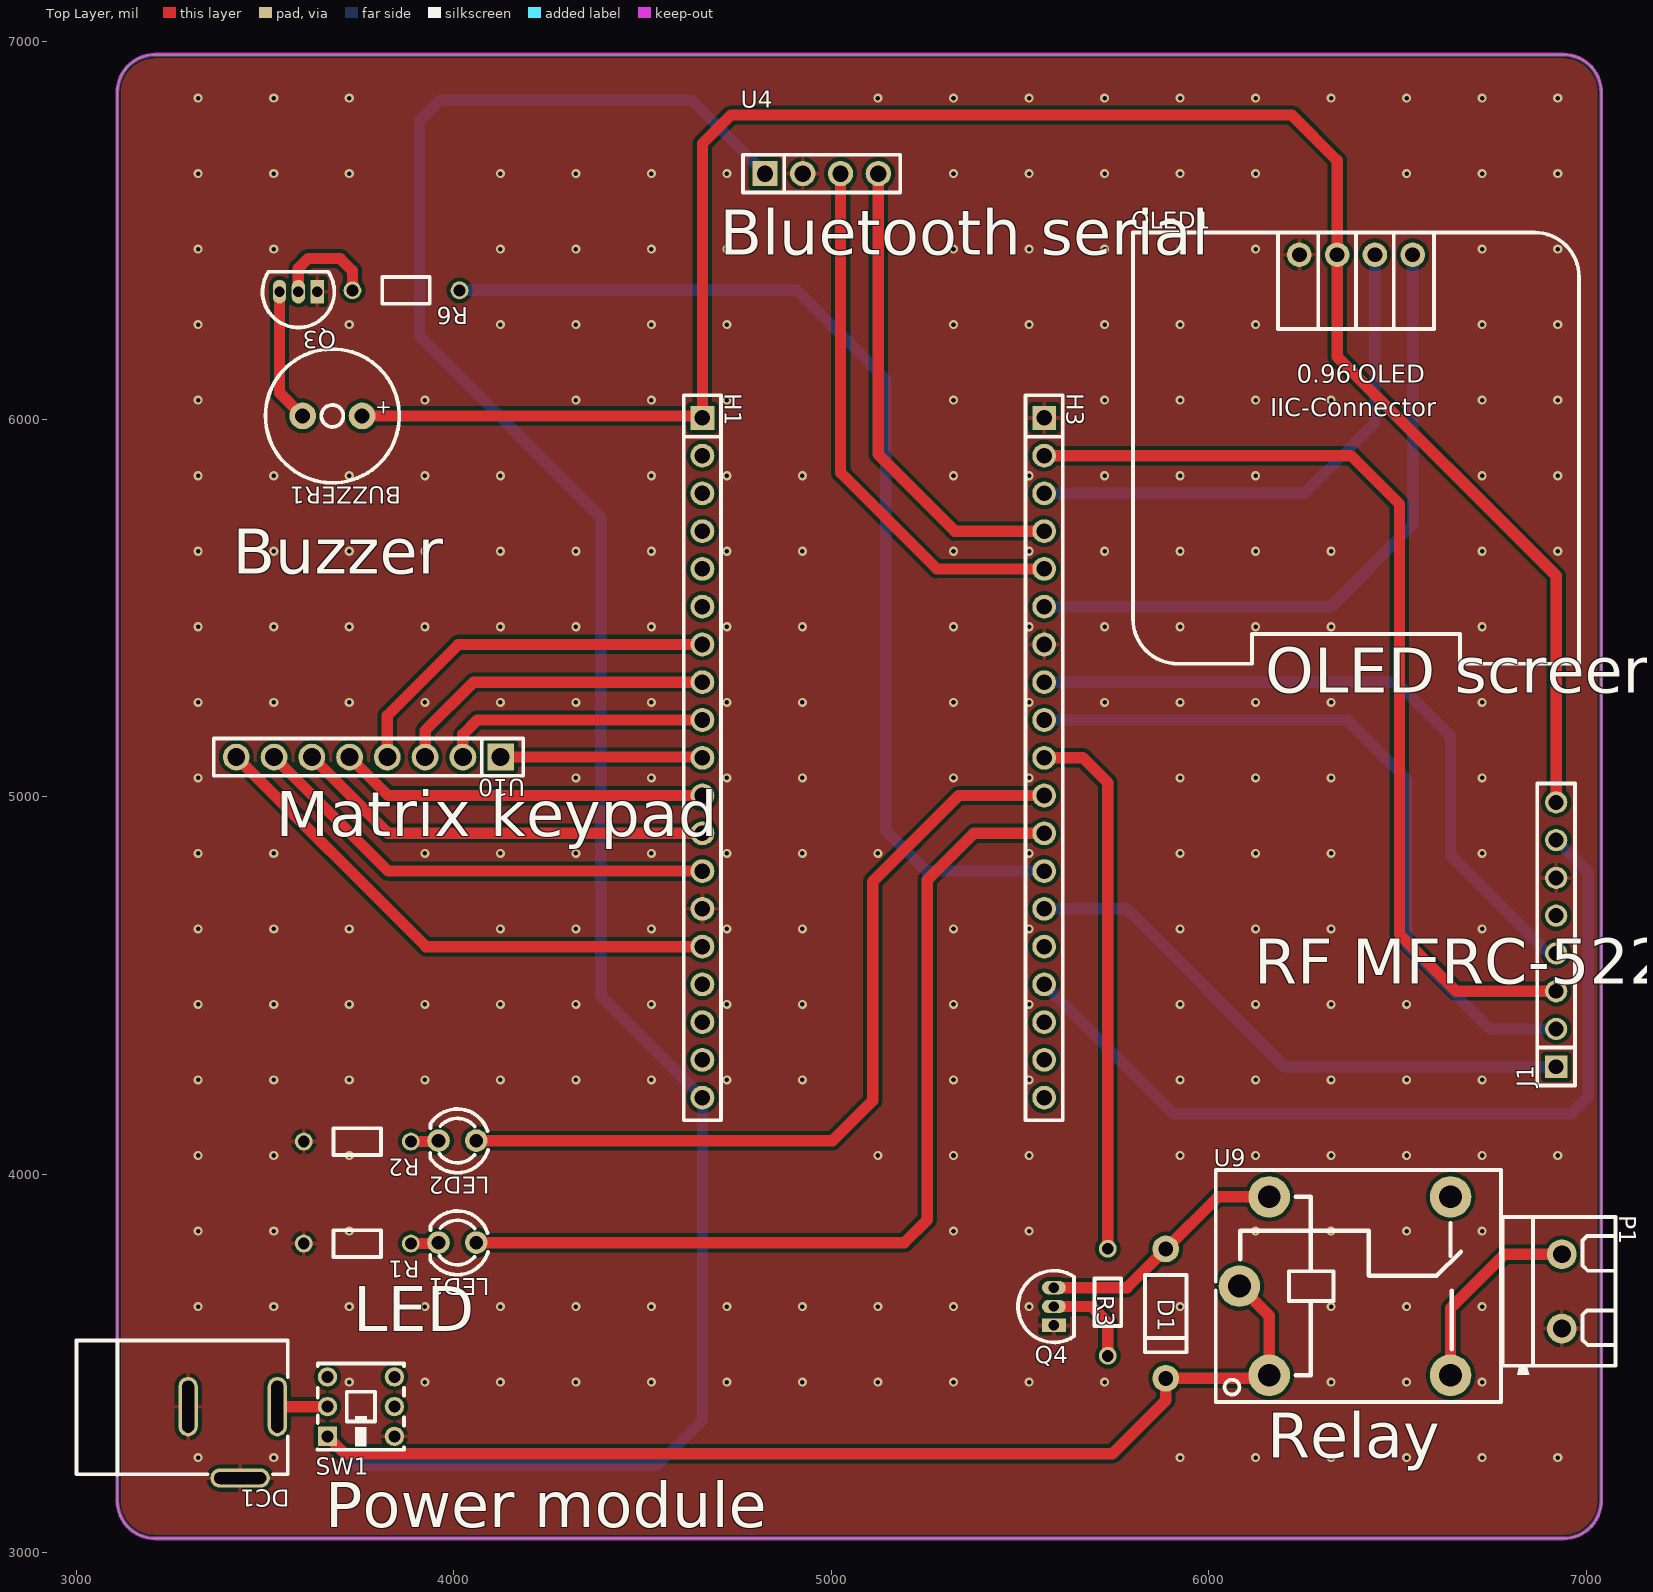
[diagram p0: Top Layer view]
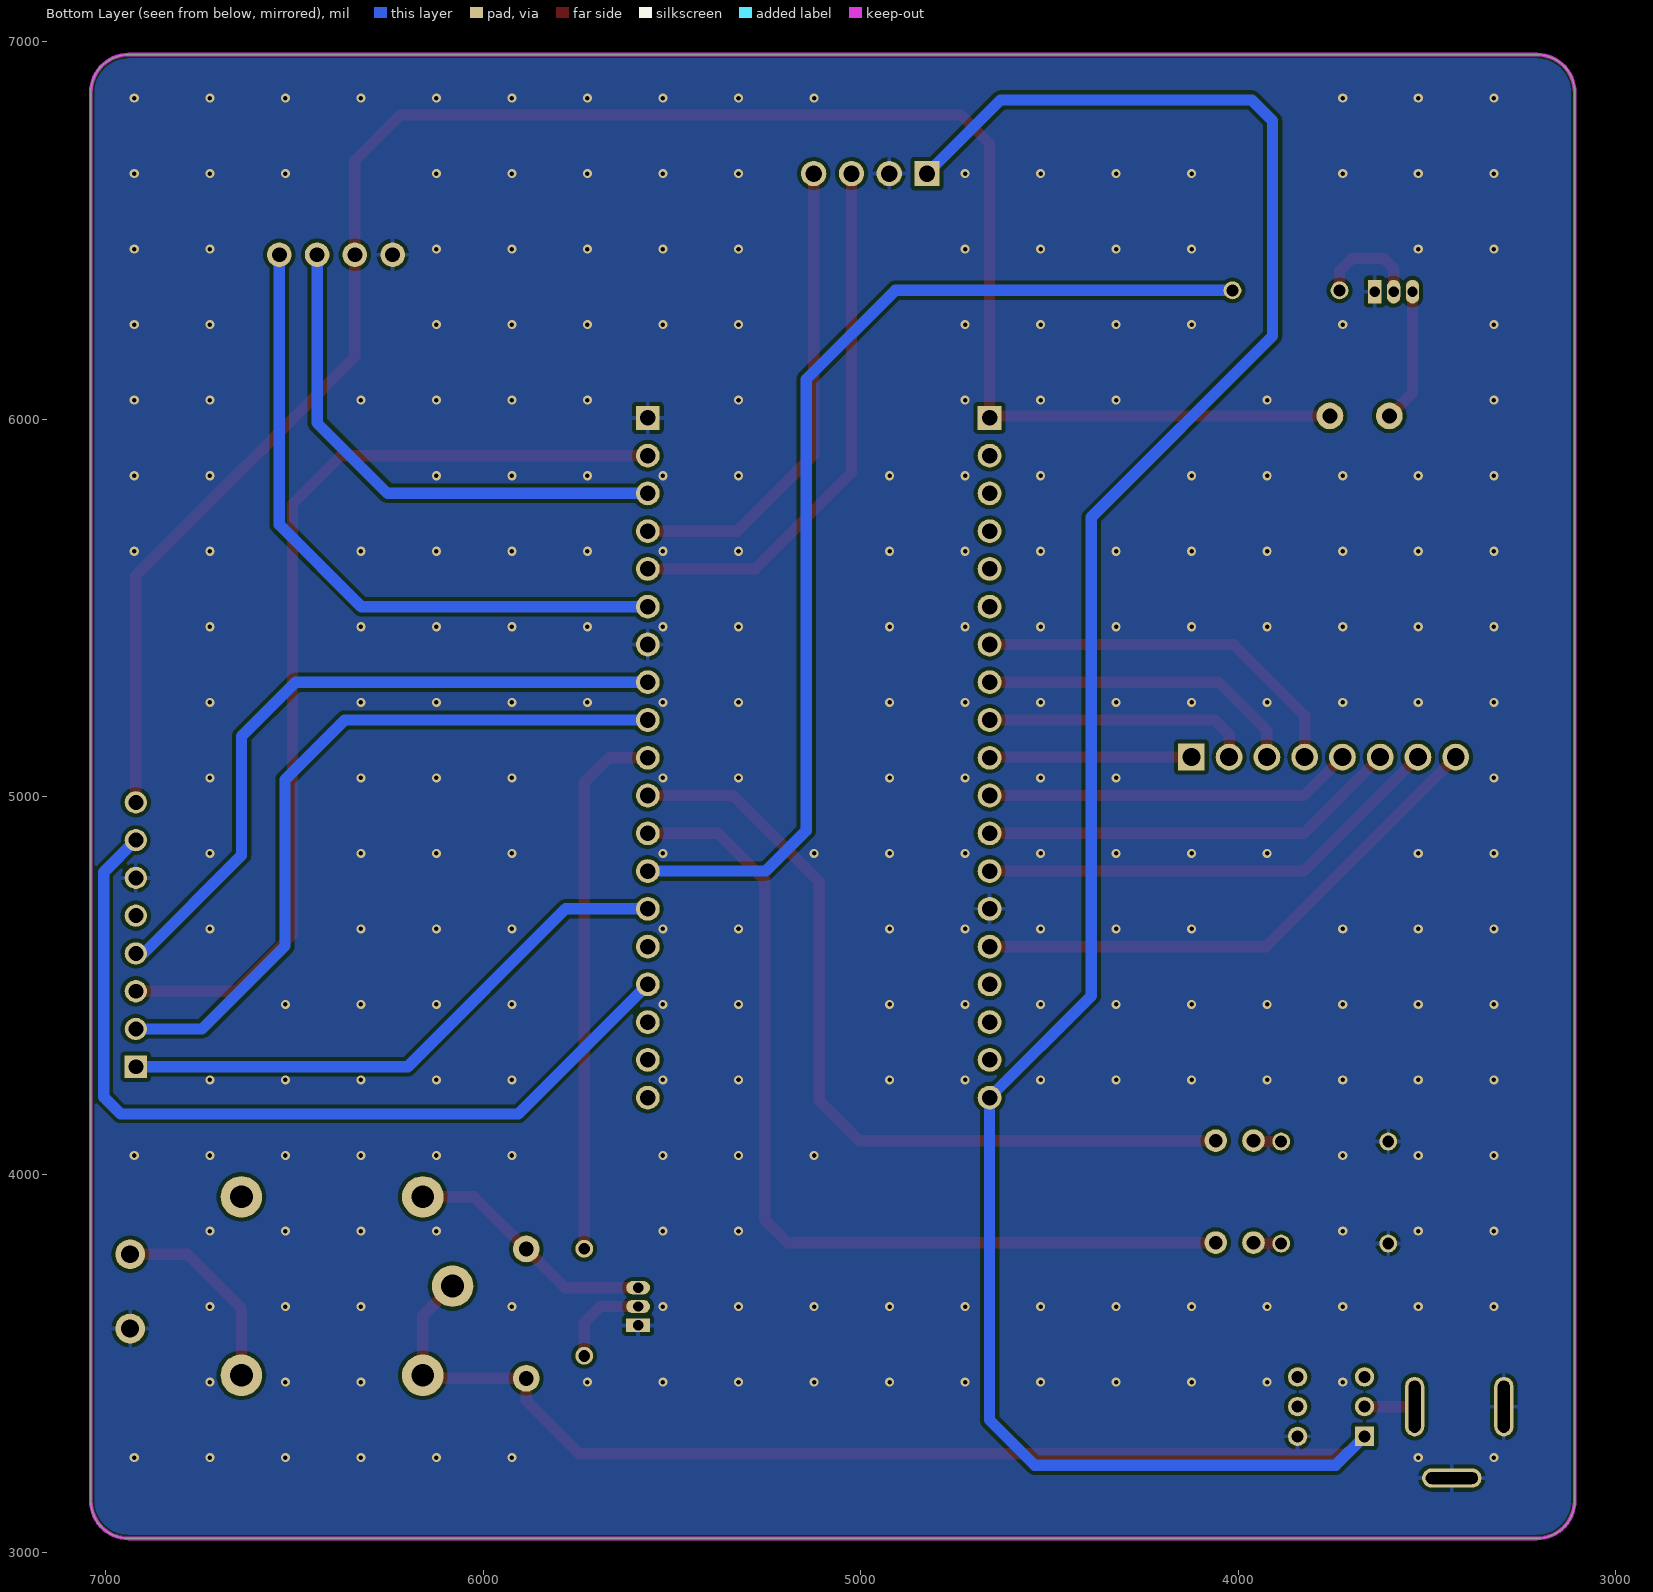
[diagram p1: Bottom Layer view, seen from below]
# Altium PCB MISC89084.pcbdoc
Units mil, origin at the board's own origin, x right, y up, seen from the top; angles counter-clockwise.
Board outline 3929.13 x 3929.13 mil, 2 copper layers (Top Layer, Bottom Layer), stack 62.206 mil thick; 20 components, 44 nets, 100 pads, 259 vias.

## Layer stack, top to bottom
Top Solder Mask Layer: solder mask 0.394, Dk 3.3
Top Layer: signal copper 1.379
Dielectric1: surface 59.449, FR4, Dk 4.5
Bottom Layer: signal copper 1.378
Bottom Solder Mask Layer: solder mask 0.394, Dk 3.3

## Board outline
3209.4,6965 ccw(c3209.4,6865) 3109.4,6865 3109.4,3135.87 ccw(c3209.4,3135.87) 3209.4,3035.87 6938.53,3035.87 ccw(c6938.53,3135.87) 7038.53,3135.87 7038.53,6865 ccw(c6938.53,6865) 6938.53,6965

## Design rules (kind name [scope] priority, off if disabled: settings)
BoardOutlineClearance copperThickness2oz_1 [All] p2 off: genericclearance=7.99 ignorepadtopadclearanceinfootprint=FALSE except(0: Arc-SplitContinuation Track-SplitContinuation SMDPad-SplitContinuation THPad-SplitContinuation Via-SplitContinuation Fill-SplitContinuation Region-SplitContinuation Poly-SplitContinuation Text-SplitContinuation Hole-SplitContinuation; 5.98: Arc-CutoutEdge Track-CutoutEdge SMDPad-CutoutEdge THPad-CutoutEdge Via-CutoutEdge Text-CutoutEdge; 6.9: Hole-OutlineEdge Hole-CutoutEdge; 10: Poly-OutlineEdge Poly-CutoutEdge; 11.81: Arc-OutlineEdge Track-OutlineEdge SMDPad-OutlineEdge THPad-OutlineEdge Via-OutlineEdge Fill-OutlineEdge Region-OutlineEdge Text-OutlineEdge Fill-CutoutEdge Region-CutoutEdge)
BoardOutlineClearance Plane_innerPlane_1 [All] p4 off: genericclearance=4.02 ignorepadtopadclearanceinfootprint=FALSE except(0: Arc-SplitContinuation Track-SplitContinuation SMDPad-SplitContinuation THPad-SplitContinuation Via-SplitContinuation Fill-SplitContinuation Region-SplitContinuation Poly-SplitContinuation Text-SplitContinuation Hole-SplitContinuation; 5.98: Arc-CutoutEdge Track-CutoutEdge SMDPad-CutoutEdge THPad-CutoutEdge Via-CutoutEdge Text-CutoutEdge; 6.9: Hole-OutlineEdge Hole-CutoutEdge; 10: Poly-OutlineEdge Poly-CutoutEdge; 11.81: Arc-OutlineEdge Track-OutlineEdge SMDPad-OutlineEdge THPad-OutlineEdge Via-OutlineEdge Fill-OutlineEdge Region-OutlineEdge Text-OutlineEdge Fill-CutoutEdge Region-CutoutEdge)
BoardOutlineClearance Copper_copperRegion_1 [All] p6 off: genericclearance=4.02 ignorepadtopadclearanceinfootprint=FALSE except(0: Arc-SplitContinuation Track-SplitContinuation SMDPad-SplitContinuation THPad-SplitContinuation Via-SplitContinuation Fill-SplitContinuation Region-SplitContinuation Poly-SplitContinuation Text-SplitContinuation Hole-SplitContinuation; 5.98: Arc-CutoutEdge Track-CutoutEdge SMDPad-CutoutEdge THPad-CutoutEdge Via-CutoutEdge Text-CutoutEdge; 6.9: Hole-OutlineEdge Hole-CutoutEdge; 10: Poly-OutlineEdge Poly-CutoutEdge; 11.81: Arc-OutlineEdge Track-OutlineEdge SMDPad-OutlineEdge THPad-OutlineEdge Via-OutlineEdge Fill-OutlineEdge Region-OutlineEdge Text-OutlineEdge Fill-CutoutEdge Region-CutoutEdge)
BoardOutlineClearance copperThickness1oz_1 [All] p8: genericclearance=4.02 ignorepadtopadclearanceinfootprint=FALSE except(0: Arc-SplitContinuation Track-SplitContinuation SMDPad-SplitContinuation THPad-SplitContinuation Via-SplitContinuation Fill-SplitContinuation Region-SplitContinuation Poly-SplitContinuation Text-SplitContinuation Hole-SplitContinuation; 5.98: Arc-CutoutEdge Track-CutoutEdge SMDPad-CutoutEdge THPad-CutoutEdge Via-CutoutEdge Text-CutoutEdge; 6.9: Hole-OutlineEdge Hole-CutoutEdge; 10: Poly-OutlineEdge Poly-CutoutEdge; 11.81: Arc-OutlineEdge Track-OutlineEdge SMDPad-OutlineEdge THPad-OutlineEdge Via-OutlineEdge Fill-OutlineEdge Region-OutlineEdge Text-OutlineEdge Fill-CutoutEdge Region-CutoutEdge)
Clearance copperThickness2oz [All] p1 off: gap=7.99 ignorepadtopadclearanceinfootprint=FALSE except(5.98: SMDPad-Track SMDPad-SMDPad THPad-Track SMDPad-THPad THPad-THPad Track-Via SMDPad-Via THPad-Via Via-Via Fill-SMDPad Region-SMDPad Fill-THPad Region-THPad Fill-Via Region-Via Fill-Fill Fill-Region Region-Region Arc-Track Arc-SMDPad Arc-THPad Arc-Via Fill-Arc Region-Arc Arc-Arc Text-Track SMDPad-Text Text-THPad Text-Via Fill-Text Region-Text Arc-Text Text-Text; 6.9: Hole-Track Hole-SMDPad Hole-THPad Hole-Via Fill-Hole Region-Hole Hole-Arc Hole-Text; 10: Poly-Track Poly-SMDPad Poly-THPad Poly-Via Poly-Fill Poly-Region Poly-Poly Poly-Arc Poly-Text Poly-Hole; 11.81: Fill-Track Region-Track)
Clearance Plane_innerPlane [All] p3 off: gap=4.02 ignorepadtopadclearanceinfootprint=FALSE except(5.98: SMDPad-Track SMDPad-SMDPad THPad-Track SMDPad-THPad THPad-THPad Track-Via SMDPad-Via THPad-Via Via-Via Fill-SMDPad Region-SMDPad Fill-THPad Region-THPad Fill-Via Region-Via Fill-Fill Fill-Region Region-Region Arc-Track Arc-SMDPad Arc-THPad Arc-Via Fill-Arc Region-Arc Arc-Arc Text-Track SMDPad-Text Text-THPad Text-Via Fill-Text Region-Text Arc-Text Text-Text; 6.9: Hole-Track Hole-SMDPad Hole-THPad Hole-Via Fill-Hole Region-Hole Hole-Arc Hole-Text; 10: Poly-Track Poly-SMDPad Poly-THPad Poly-Via Poly-Fill Poly-Region Poly-Poly Poly-Arc Poly-Text Poly-Hole; 11.81: Fill-Track Region-Track)
Clearance Copper_copperRegion [All] p5 off: gap=4.02 ignorepadtopadclearanceinfootprint=FALSE except(5.98: SMDPad-Track SMDPad-SMDPad THPad-Track SMDPad-THPad THPad-THPad Track-Via SMDPad-Via THPad-Via Via-Via Fill-SMDPad Region-SMDPad Fill-THPad Region-THPad Fill-Via Region-Via Fill-Fill Fill-Region Region-Region Arc-Track Arc-SMDPad Arc-THPad Arc-Via Fill-Arc Region-Arc Arc-Arc Text-Track SMDPad-Text Text-THPad Text-Via Fill-Text Region-Text Arc-Text Text-Text; 6.9: Hole-Track Hole-SMDPad Hole-THPad Hole-Via Fill-Hole Region-Hole Hole-Arc Hole-Text; 10: Poly-Track Poly-SMDPad Poly-THPad Poly-Via Poly-Fill Poly-Region Poly-Poly Poly-Arc Poly-Text Poly-Hole; 11.81: Fill-Track Region-Track)
Clearance copperThickness1oz [All] p7: gap=4.02 ignorepadtopadclearanceinfootprint=FALSE except(5.98: SMDPad-Track SMDPad-SMDPad THPad-Track SMDPad-THPad THPad-THPad Track-Via SMDPad-Via THPad-Via Via-Via Fill-SMDPad Region-SMDPad Fill-THPad Region-THPad Fill-Via Region-Via Fill-Fill Fill-Region Region-Region Arc-Track Arc-SMDPad Arc-THPad Arc-Via Fill-Arc Region-Arc Arc-Arc Text-Track SMDPad-Text Text-THPad Text-Via Fill-Text Region-Text Arc-Text Text-Text; 6.9: Hole-Track Hole-SMDPad Hole-THPad Hole-Via Fill-Hole Region-Hole Hole-Arc Hole-Text; 10: Poly-Track Poly-SMDPad Poly-THPad Poly-Via Poly-Fill Poly-Region Poly-Poly Poly-Arc Poly-Text Poly-Hole; 11.81: Fill-Track Region-Track)
DiffPairsRouting differentialPair [All] p1: maxlimit=6 minlimit=6 mostfreqgap=6 toplayer_minwidth=5 toplayer_prefwidth=10 toplayer_maxwidth=100 toplayer_mingap=6 toplayer_prefgap=6 toplayer_maxgap=6 bottomlayer_minwidth=5 bottomlayer_prefwidth=10 bottomlayer_maxwidth=100 bottomlayer_mingap=6 bottomlayer_prefgap=6 bottomlayer_maxgap=6 maxuncoupledlength=10
HoleToHoleClearance otherClearance [All] p1: gap=11.81 allowstackedmicrovias=TRUE
Length netLength [All] p1: minlimit=0 maxlimit=0
PasteMaskExpansion pasteMaskExpansion [All] p1: expansion=0
PlaneConnect innerPlane [All] p1: planeconnectstyle=Relief reliefexpansion=20 reliefentries=4 reliefconductorwidth=10 reliefairgap=10
PolygonConnect copperRegion [All] p1: connectstyle=Relief reliefconductorwidth=10 reliefentries=4 polygonreliefangle="90 Angle" airgapwidth=10 via.connectstyle=Relief via.reliefconductorwidth=10 via.reliefentries=4 via.polygonreliefangle="90 Angle" via.airgapwidth=10
RoutingVias viaSize [All] p1: holewidth=12.01 width=24.02 viastyle="Through Hole" minholewidth=11.81 minwidth=19.68 maxholewidth=248.03 maxwidth=393.7
SolderMaskExpansion solderMaskExpansion [IsVia] p1: expansion=-1000 istentingtop=TRUE
SolderMaskExpansion solderMaskExpansion [All] p2: expansion=2 istentingtop=FALSE
Width copperThickness2oz_2 [All] p1 off: maxlimit=100 minlimit=8 preferedwidth=10
Width copperThickness1oz_2 [All] p2: maxlimit=100 minlimit=5 preferedwidth=10

## Components (designator, comment, footprint, x,y, rotation, side; value= is the part's Value field where it differs from the comment)
BUZZER1 "2.7kHz" BUZ-TH_BD9.0-P4.00-D0.6-FD 3678.79,6008.3 r180 top
D1 "" DO_1N4007 5885.61,3631.17 r90 top
DC1 "" DC-2.0 3410,3395.3 r180 top
H1 "C2897382" HDR-TH_19P-P2.54-V-F 4658.71,5103.13 r270 top
H3 "C2897382" HDR-TH_19P-P2.54-V-F 5563.71,5103.13 r270 top
J1 "" HDR-TH_8P-P2.54-V-M 6919.4,4635 r90 top
LED1 "" LED_TH-3mm 4009.8,3819.31 r180 top
LED2 "" LED_TH-3mm 4009.8,4089.31 r180 top
OLED1 "" 0.96OLED_4P 6389.4,6435 r0 top
P1 "KF301-2P terminal block" CONN-TH_XY301V-A-5.0-2P 6934.4,3690 r270 top
Q3 "" S8050_TO_92 3588.79,6337.3 r180 top
Q4 "" S8050_TO_92 5589.4,3650 r90 top
R1 "220Ω" Res_1/8W 3744.81,3819.31 r180 top
R2 "220Ω" Res_1/8W 3744.81,4089.31 r180 top
R3 "1K" Res_1/8W 5729.62,3661.17 r270 top
R6 "1K" Res_1/8W 3873.78,6343.3 r180 top
SW1 "5.8 WSPT" SW-TH_6P-L5.8-W5.8-P2.00-LS4.5-TL_K8-5851E-L1 3754.4,3385 r90 top
U4 "" HDR-TH_4P-P2.54-V-F 4974.4,6650 r0 top
U9 "SRD-12VDC-SL-C" RELAY-TH_SRD-XXVDC-XL-C 6360.23,3704.17 r0 top
U10 "" HDR-TH_8P-P2.54-V-F-1 3774.4,5105 r180 top

## Footprints (in the part's own frame and the unit in brackets; to place one, negate y for a bottom-side part, rotate by r counter-clockwise, add the part's x,y. Pads: shape width x height; smd on the part's side, far side on the other; paste and mask are expansions set on the pad)
0.96OLED_4P [mm]
  round 1.65 hole 1 copper offset 0,0: 1(-3.81,-0.001) 2(-1.27,0.002) 3(1.27,0.002) 4(3.81,0.002)
  silkscreen extent -15,-27.5 15,1.5
BUZ-TH_BD9.0-P4.00-D0.6-FD [mm]
  round 1.8 hole 1: 1(-2,0) 2(2,0)
  silkscreen extent -4.5,-4.5 4.5,4.5
CONN-TH_XY301V-A-5.0-2P [mm]
  round 2 hole 1.2: 1(-2.5,0) 2(2.5,0)
  silkscreen extent -5,-4 5.6,3.6
DC-2.0 [mil]
  oval 157.5x51.2 hole 31.5 slot 137.8 at 0 deg paste+0 mask+2: 2(-24.7,199.5)
  oval 51.2x157.5 hole 31.5 slot 137.8 at 90 deg paste+0 mask+2: 3(113.1,10.5) 4(-123.1,10.5)
  silkscreen extent -151,-165 408,190
DO_1N4007 [mm]
  round 1.8 hole 1 paste+0 mask+0.051: 1(-4.35,0) 2(4.35,0)
  silkscreen extent -2.6,-1.4 2.6,1.4
HDR-TH_4P-P2.54-V-F [mm]
  rect 1.7x1.7 hole 1.1: 1(-3.81,0)
  round 1.7 hole 1.1: 2(-1.27,0) 3(1.27,0) 4(3.81,0)
  silkscreen extent -5.29,-1.27 5.29,1.27
HDR-TH_8P-P2.54-V-F-1 [mm]
  rect 1.8x1.8 hole 1.2: 1(-8.89,0)
  round 1.8 hole 1.2: 2(-6.35,0) 3(-3.81,0) 4(-1.27,0) 5(1.27,0) 6(3.81,0) 7(6.35,0) 8(8.89,0)
  silkscreen extent -10.41,-1.25 10.41,1.25
HDR-TH_8P-P2.54-V-M [mm]
  rect 1.5x1.5 hole 1: 1(-8.89,0)
  round 1.5 hole 1: 2(-6.35,0) 3(-3.81,0) 4(-1.27,0) 5(1.27,0) 6(3.81,0) 7(6.35,0) 8(8.89,0)
  silkscreen extent -10.16,-1.27 10.16,1.27
HDR-TH_19P-P2.54-V-F [mm]
  rect 1.6x1.6 hole 1.05: 1(-22.86,0)
  round 1.6 hole 1.05: 2(-20.32,0) 3(-17.78,0) 4(-15.24,0) 5(-12.7,0) 6(-10.16,0) 7(-7.62,0) 8(-5.08,0) 9(-2.54,0) 10(0,0) 11(2.54,0) 12(5.08,0) 13(7.62,0) 14(10.16,0) 15(12.7,0) 16(15.24,0) 17(17.78,0) 18(20.32,0) 19(22.86,0)
  silkscreen extent -24.38,-1.25 24.38,1.25
LED_TH-3mm [mil]
  round 60 hole 36 paste+0 mask+2: 1(-50,0) 2(50,0)
  silkscreen extent -81,-84 72,85
RELAY-TH_SRD-XXVDC-XL-C [mil]
  round 110 hole 60: 1(-200.79,-236.22) 2(279.52,-236.2) 3(279.53,236.2) 4(-200.79,236.22) 5(-279.53,0)
  silkscreen extent -342,-307 413,307
Res_1/8W [mil]
  round 47.2 hole 31.5 paste+0 mask+2: 1(-141.7,2.48) 2(141.7,2.48)
  silkscreen extent -63,-33 63,38
S8050_TO_92 [mil]
  rect 35.4x63 hole 27.6 paste+0 mask+2: 1(-50,0)
  oval 35.4x63 hole 27.6 paste+0 mask+2: 2(0,0) 3(50,0)
  silkscreen extent -95,-53 95,95
SW-TH_6P-L5.8-W5.8-P2.00-LS4.5-TL_K8-5851E-L1 [mm]
  rect 1.3x1.3 hole 0.8 paste+0 mask+0.05: 1(-2,2.25)
  round 1.3 hole 0.8 paste+0 mask+0.05: 2(0,2.25) 3(2,2.25) 4(-2,-2.25) 5(0,-2.25) 6(2,-2.25)
  silkscreen extent -2.9,-2.9 2.9,2.92

## Via types
v1: diameter 24.02, hole 12, Top Layer to Bottom Layer, 259 vias

## Nets (pads, with @x,y where several pads share a name; then routed paths per layer and width w, separated by ;. In a path a pad name is that pad's centre, name@x,y a point inside that pad or via, vN(x,y) a via of type N, cw(c..) or ccw(c..) an arc to the next point about the centre after c; other vN are vias at no path point)
$1N1877: BUZZER1.2 Q3.3 | length 354.4
  Top Layer w30: Q3.3 3538.79,6069.56 BUZZER1.2
$1N2018: Q3.2 R6.2 | length 281
  Top Layer w30: Q3.2 3588.79,6399.39 3614.4,6425 3699.4,6425 3732.08,6392.32 R6.2
$1N4284: DC1.4 SW1.2 | length 132.8
  Top Layer w30: DC1.4 3665.61,3384.8 SW1.2
$1N4728: P1.1 U9.2 | length 531.3
  Top Layer w30: U9.2 6639.76,3645.36 6782.82,3788.43 P1.1
$1N4736: D1.2 Q4.3 U9.4 | length 669.6
  Top Layer w30: Q4.3 5783.18,3700 D1.2 6023.57,3940.39 U9.4
$1N5006: Q4.2 R3.2 | length 248.2
  Top Layer w30: Q4.2 5689.4,3650 5732.09,3607.3 R3.2
$1N5098: LED1.2 R1.1 | length 74.3
  Top Layer w30: R1.1 3957.32,3816.84 LED1.2
$1N5101: LED2.2 R2.1 | length 74.3
  Top Layer w30: R2.1 3957.32,4086.84 LED2.2
+5V: D1.1 H1.19 SW1.1 U4.1 U9.1 U9.5 | length 8745.9
  Top Layer w30: SW1.1 3712.39,3259.69 3862.27,3259.69 3862.58,3260 5744.4,3260 5885.61,3401.22 D1.1 6151.4,3459.91 U9.1 6159.44,3625.43 U9.5
  Bottom Layer w30: SW1.1 3742.08,3230 4539.4,3230 4658.71,3349.32 H1.19 4389.4,4472.44 4389.4,5740 3909.4,6220 3909.4,6790 3964.4,6845 4629.4,6845 U4.1
BEEP: H3.13 R6.1 | length 2885.2
  Bottom Layer w30: R6.1 4908.57,6340.82 5144.4,6105 5144.4,4910 5251.27,4803.13 H3.13
CLK: H3.19
CMD: H1.18
EN: H1.2
GND: DC1.2 DC1.3 H1.14 H3.1 H3.7 J1.6 OLED1.1 P1.2 Q3.1 Q4.1 R1.2 R2.2 SW1.4 U4.2
  other v1: 3323.5,3249.97 3523.5,3249.97 5923.5,3249.97 6123.5,3249.97 6323.5,3249.97 6523.5,3249.97 6723.5,3249.97 6923.5,3249.97 3723.5,3449.97 3923.5,3449.97 4123.5,3449.97 4323.5,3449.97 4523.5,3449.97 4723.5,3449.97 4923.5,3449.97 5123.5,3449.97 5323.5,3449.97 5523.5,3449.97 5723.5,3449.97 6323.5,3449.97 6523.5,3449.97 6723.5,3449.97 3323.5,3649.97 3523.5,3649.97 3723.5,3649.97 3923.5,3649.97 4123.5,3649.97 4323.5,3649.97 4523.5,3649.97 4723.5,3649.97 4923.5,3649.97 5123.5,3649.97 5323.5,3649.97 5523.5,3649.97 5923.5,3649.97 6323.5,3649.97 6523.5,3649.97 6723.5,3649.97 3323.5,3849.97 3523.5,3849.97 3723.5,3849.97 5323.5,3849.97 5523.5,3849.97 6123.5,3849.97 6323.5,3849.97 6523.5,3849.97 6723.5,3849.97 3323.5,4049.97 3523.5,4049.97 3723.5,4049.97 5123.5,4049.97 5323.5,4049.97 5523.5,4049.97 5923.5,4049.97 6123.5,4049.97 6323.5,4049.97 6523.5,4049.97 6723.5,4049.97 6923.5,4049.97 3323.5,4249.97 3523.5,4249.97 3723.5,4249.97 3923.5,4249.97 4123.5,4249.97 4323.5,4249.97 4523.5,4249.97 4723.5,4249.97 4923.5,4249.97 5323.5,4249.97 5523.5,4249.97 5923.5,4249.97 6123.5,4249.97 6323.5,4249.97 6523.5,4249.97 6723.5,4249.97 3323.5,4449.97 3523.5,4449.97 3723.5,4449.97 3923.5,4449.97 4123.5,4449.97 4323.5,4449.97 4523.5,4449.97 4723.5,4449.97 4923.5,4449.97 5323.5,4449.97 5523.5,4449.97 5923.5,4449.97 6123.5,4449.97 6323.5,4449.97 6523.5,4449.97 3323.5,4649.97 3523.5,4649.97 3723.5,4649.97 4123.5,4649.97 4323.5,4649.97 4523.5,4649.97 4723.5,4649.97 4923.5,4649.97 5323.5,4649.97 5523.5,4649.97 5923.5,4649.97 6123.5,4649.97 6323.5,4649.97 6723.5,4649.97 3323.5,4849.97 3523.5,4849.97 3923.5,4849.97 4123.5,4849.97 4323.5,4849.97 4523.5,4849.97 4723.5,4849.97 4923.5,4849.97 5123.5,4849.97 5523.5,4849.97 5923.5,4849.97 6123.5,4849.97 6323.5,4849.97 6723.5,4849.97 3323.5,5049.97 4323.5,5049.97 4523.5,5049.97 4723.5,5049.97 4923.5,5049.97 5323.5,5049.97 5523.5,5049.97 5923.5,5049.97 6123.5,5049.97 6323.5,5049.97 6723.5,5049.97 3323.5,5249.97 3523.5,5249.97 3723.5,5249.97 3923.5,5249.97 4123.5,5249.97 4323.5,5249.97 4523.5,5249.97 4723.5,5249.97 4923.5,5249.97 5323.5,5249.97 5523.5,5249.97 5723.5,5249.97 5923.5,5249.97 6123.5,5249.97 6323.5,5249.97 6723.5,5249.97 3323.5,5449.97 3523.5,5449.97 3723.5,5449.97 3923.5,5449.97 4123.5,5449.97 4323.5,5449.97 4523.5,5449.97 4723.5,5449.97 4923.5,5449.97 5323.5,5449.97 5523.5,5449.97 5723.5,5449.97 5923.5,5449.97 6123.5,5449.97 6323.5,5449.97 6723.5,5449.97 3323.5,5649.97 3523.5,5649.97 3723.5,5649.97 3923.5,5649.97 4123.5,5649.97 4323.5,5649.97 4523.5,5649.97 4723.5,5649.97 4923.5,5649.97 5323.5,5649.97 5523.5,5649.97 5723.5,5649.97 5923.5,5649.97 6123.5,5649.97 6323.5,5649.97 6723.5,5649.97 6923.5,5649.97 3323.5,5849.97 3523.5,5849.97 3723.5,5849.97 3923.5,5849.97 4123.5,5849.97 4523.5,5849.97 4723.5,5849.97 4923.5,5849.97 5323.5,5849.97 5523.5,5849.97 5723.5,5849.97 5923.5,5849.97 6123.5,5849.97 6723.5,5849.97 6923.5,5849.97 3323.5,6049.97 3923.5,6049.97 4323.5,6049.97 4523.5,6049.97 4723.5,6049.97 5323.5,6049.97 5723.5,6049.97 5923.5,6049.97 6123.5,6049.97 6323.5,6049.97 6723.5,6049.97 6923.5,6049.97 3323.5,6249.97 3723.5,6249.97 4123.5,6249.97 4323.5,6249.97 4523.5,6249.97 4723.5,6249.97 5323.5,6249.97 5523.5,6249.97 5723.5,6249.97 5923.5,6249.97 6123.5,6249.97 6723.5,6249.97 6923.5,6249.97 3323.5,6449.97 3523.5,6449.97 4123.5,6449.97 4323.5,6449.97 4523.5,6449.97 4723.5,6449.97 5323.5,6449.97 5523.5,6449.97 5723.5,6449.97 5923.5,6449.97 6123.5,6449.97 6723.5,6449.97 6923.5,6449.97 3323.5,6649.97 3523.5,6649.97 3723.5,6649.97 4123.5,6649.97 4323.5,6649.97 4523.5,6649.97 4723.5,6649.97 5323.5,6649.97 5523.5,6649.97 5723.5,6649.97 5923.5,6649.97 6123.5,6649.97 6523.5,6649.97 6723.5,6649.97 6923.5,6649.97 3323.5,6849.97 3523.5,6849.97 3723.5,6849.97 5123.5,6849.97 5323.5,6849.97 5523.5,6849.97 5723.5,6849.97 5923.5,6849.97 6123.5,6849.97 6323.5,6849.97 6523.5,6849.97 6723.5,6849.97 6923.5,6849.97
MFR_MISO: H3.8 J1.4 | length 1837.7
  Bottom Layer w30: H3.8 6496.27,5303.13 6639.4,5160 6639.4,4845 6899.4,4585 J1.4
MFR_MOSI: H3.2 J1.3 | length 2610.9
  Top Layer w30: H3.2 6376.27,5903.13 6504.4,5775 6504.4,4635 6654.4,4485 J1.3
MFR_RST: H3.16 J1.7 | length 2316.7
  Bottom Layer w30: H3.16 5906.84,4160 6959.4,4160 7004.4,4205 7004.4,4800 J1.7
MFR_SCK: H3.9 J1.2 | length 1952.3
  Bottom Layer w30: H3.9 6366.27,5203.13 6524.4,5045 6524.4,4605 6744.4,4385 J1.2
MFR_SDA: H3.14 J1.1 | length 1528.9
  Bottom Layer w30: H3.14 5781.27,4703.13 6199.4,4285 J1.1
P2: H3.15
P5: H3.10 R3.1 | length 1430.1
  Top Layer w30: H3.10 5666.27,5103.13 5732.09,5037.3 R3.1
P12: H1.13 U10.7 | length 1259.4
  Top Layer w30: U10.7 3826.27,4803.13 H1.13
P13: H1.15 U10.8 | length 1442.2
  Top Layer w30: U10.8 3926.27,4603.13 H1.15
P14: H1.12 U10.6 | length 1117.9
  Top Layer w30: U10.6 3826.27,4903.13 H1.12
P16: H3.12 LED1.1 | length 2480.1
  Top Layer w30: LED1.1 5193.71,3819.31 5254.4,3880 5254.4,4780 5377.53,4903.13 H3.12
P17: H3.11 LED2.1 | length 2222.2
  Top Layer w30: LED2.1 5003.71,4089.31 5109.4,4195 5109.4,4775 5337.53,5003.13 H3.11
P21: H3.6 OLED1.4 | length 1780.6
  Bottom Layer w30: H3.6 6322.53,5503.13 6539.4,5720 OLED1.4@6539.4,6435.05
P22: H3.3 OLED1.3 | length 1398.1
  Bottom Layer w30: H3.3 6252.53,5803.13 6439.4,5990 OLED1.3@6439.4,6435.05
P25: H1.9 U10.2 | length 710.1
  Top Layer w30: U10.2 4024.4,5165 4062.53,5203.13 H1.9
P26: H1.10 U10.1 | length 535.1
  Top Layer w30: U10.1 4656.84,5105 H1.10
P27: H1.11 U10.5 | length 976.5
  Top Layer w30: U10.5 3826.27,5003.13 H1.11
P32: H1.7 U10.4 | length 1022.2
  Top Layer w30: U10.4 3824.4,5215 4012.53,5403.13 H1.7
P33: H1.8 U10.3 | length 857.4
  Top Layer w30: U10.3 3924.4,5175 4052.53,5303.13 H1.8
P34: H1.5
P35: H1.6
RX0: H3.5 U4.3 | length 1436.7
  Top Layer w30: U4.3 5024.4,5858.26 5279.53,5603.13 H3.5
SD0: H3.18
SD1: H3.17
SD2: H1.16
SD3: H1.17
SVN: H1.4
SVP: H1.3
TX0: H3.4 U4.4 | length 1267.4
  Top Layer w30: U4.4 5124.4,5905.95 5327.22,5703.13 H3.4
VCC: BUZZER1.1 H1.1 J1.8 OLED1.2 | length 5331.5
  Top Layer w30: BUZZER1.1 4653.54,6008.3 H1.1 4658.71,6729.32 4734.4,6805 6219.4,6805 6339.4,6685 6339.4,6435.05 6339.4,6165 6919.4,5585 J1.8
pads on no net: J1.5 SW1.3 SW1.5 SW1.6 U9.3

## Polygon pours and split planes (outlines as drawn)
GND on Top Layer (solid, remove dead copper, pour order 0): 3064.4,6980 3064.4,3000 7064.4,3000 7064.4,6980
GND on Bottom Layer (solid, remove dead copper, pour order 2): 3064.4,6985 3064.4,3010 7059.4,3010 7059.4,6985

## Keep-outs
Board Outline Layer:
  the board outline again, w10

## Silkscreen, mask and mechanical layers (free items; w line width, h text height)
Top Silkscreen Layer:
  text "Bluetooth serial" at 4704.4,6435 h120
  text "Buzzer" at 3414.4,5590 h120
  text "OLED screen" at 6149.4,5275 h120
  text "Matrix keypad" at 3529.4,4895 h120
  text "RF MFRC-522" at 6119.4,4505 h120
  text "LED" at 3734.4,3585 h120
  text "Relay" at 6154.4,3250 h120
  text "Power module" at 3659.4,3065 h120